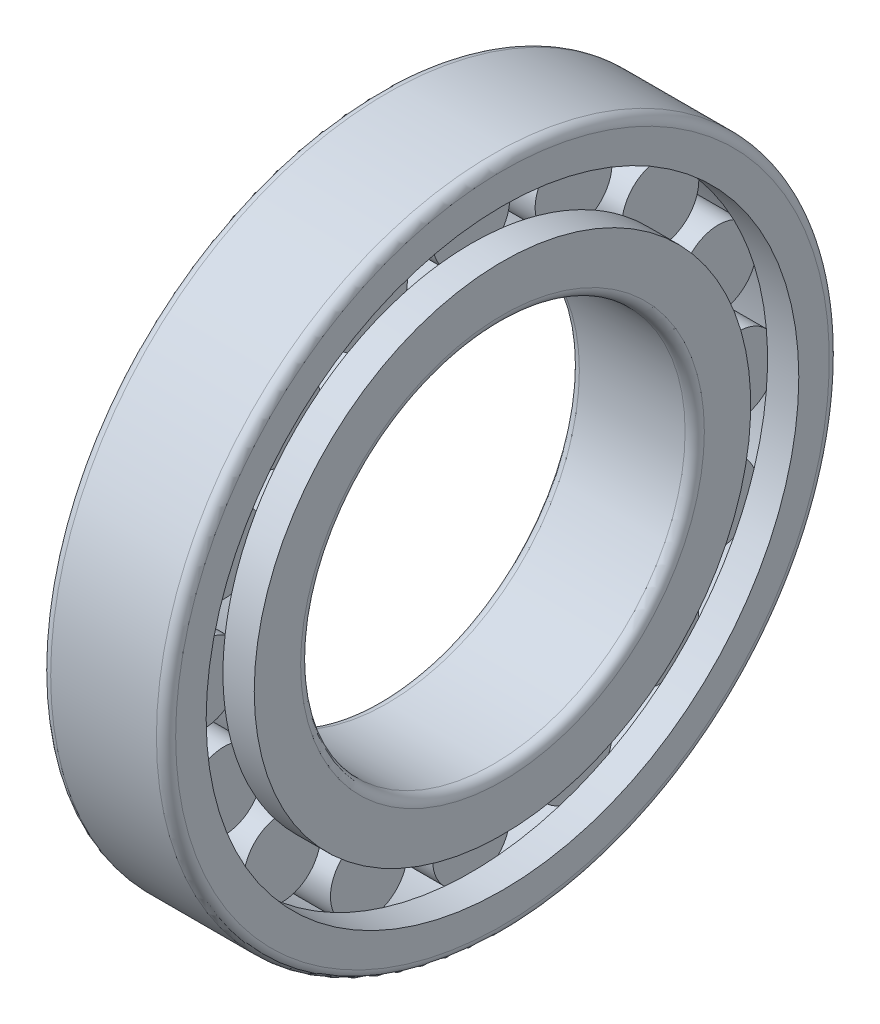
SolidWorks part; units mm, degrees
revolve "基体-旋转" add sketch "草图2" angle 360 about L0
sketch "草图2" plane through (0, 0, 0) normal (0, 0, 1) x (1, 0, 0)
  line L0 (-10.0801, 0) -> (21.9267, 0) construction
  line L1 (6.5, 47.65) -> (19.5, 47.65)
  line L2 (0, 51.65) -> (6.5, 51.65)
  line L3 (0, 51.65) -> (0, 42)
  line L4 (2, 40) -> (24, 40)
  line L5 (26, 51.65) -> (26, 42)
  line L6 (6.5, 47.65) -> (6.5, 51.65)
  line L7 (19.5, 47.65) -> (19.5, 51.65)
  line L8 (19.5, 51.65) -> (26, 51.65)
  arc A0 (24, 40) -> (26, 42) centre (24, 42) ccw
  arc A1 (0, 42) -> (2, 40) centre (2, 42) ccw
  point P13 (26, 40)
  point P16 (0, 40)
material "GCr15"
ref_plane "基准面1" through (0, 0, 0) normal (0, 0, 1) x (1, 0, 0)
ref_plane "基准面2" through (0, 0, 0) normal (0, 1, 0) x (1, 0, 0)
ref_plane "基准面3" through (0, 0, 0) normal (1, 0, 0) x (0, 0, -1)
sketch "尺寸草图" plane through (0, 0, 0) normal (0, 0, 1) x (1, 0, 0)
  line L0 (0, 0) -> (2, 0)
  line L1 (2, 0) -> (4, 0)
  line L2 (4, 0) -> (30, 0)
  line L3 (30, 0) -> (110, 0)
  line L4 (110, 0) -> (205.3, 0)
  line L5 (205.3, 0) -> (345.3, 0)
  line L7 (345.3, 0) -> (472.6, 0)
sketch "草图3" plane through (0, 0, 0) normal (0, 0, 1) x (1, 0, 0)
  line L0 (19.5, 51.65) -> (19.5, -51.65) construction
  line L2 (-1.6039, 55.65) -> (13.5036, 55.65) construction
  line L4 (6.5, 55.65) -> (19.5, 55.65)
  line L5 (6.5, 55.65) -> (6.5, 47.6499)
  line L6 (6.5, 47.6499) -> (19.5, 47.6499)
  line L7 (19.5, 55.65) -> (19.5, 47.6499)
  line L8 (6.5, -51.65) -> (6.5, 51.65) construction
revolve "凸台-旋转1" add sketch "草图3" angle 360 about L2
sketch "草图4" plane through (0, 0, 0) normal (0, 0, 1) x (1, 0, 0)
  line L0 (0, 0) -> (17.8006, 0) construction
  line L1 (-10.0801, 0) -> (21.9267, 0) construction
  line L2 (19.5, 61.65) -> (26, 61.65)
  line L3 (2, 70) -> (24, 70)
  line L4 (0, 68) -> (0, 61.65)
  line L5 (0, 61.65) -> (6.5, 61.65)
  line L6 (26, 68) -> (26, 61.65)
  line L7 (6.5, 63.65) -> (19.5, 63.65)
  line L8 (6.5, 63.65) -> (6.5, 61.65)
  line L10 (19.5, 63.65) -> (19.5, 61.65)
  arc A0 (24, 70) -> (26, 68) centre (24, 68) cw
  arc A1 (2, 70) -> (0, 68) centre (2, 68) ccw
  point P15 (26, 70)
  point P18 (0, 70)
revolve "凸台-旋转2" add sketch "草图4" angle 360 about L0
pattern_circular "阵列(圆周)1" count 16 over 360 about axis through (0, 0, 0) along (1, 0, 0) of "凸台-旋转1"
equation "\"DD@草图2\" = \"内径@尺寸草图\""
equation "\"FW@草图2\" = \"参考FW@尺寸草图\""
equation "\"D1@草图2\" = \"倒角小@尺寸草图\""
equation "\"EW@草图4\" = \"参考EW@尺寸草图\""
equation "\"D@草图4\" = \"外径@尺寸草图\""
equation "\"D2@草图4\" = \"倒角大@尺寸草图\""
equation "\"B@草图4\" = \"宽度@尺寸草图\""
equation "\"D2@草图2\" = \"B@草图4\""
equation "\"滚珠位置@草图2\" = \"D2@草图2\"/4"
equation "\"D3@草图4\" = \"D2@草图4\""
equation "\"D1@草图3\" =  ( \"EW@草图4\" - \"FW@草图2\" )  / 4 + \"FW@草图2\" / 2"
equation "\"D2@草图3\" =  0.25*( \"EW@草图4\" - \"FW@草图2\" ) +0.0001"
equation "\"D4@草图2\" = \"FW@草图2\" + 4 *\"D1@草图2\""
equation "\"D1@阵列(圆周)1\" =0.75* \"D1@草图3\" * 3.14 / \"D2@草图3\""
